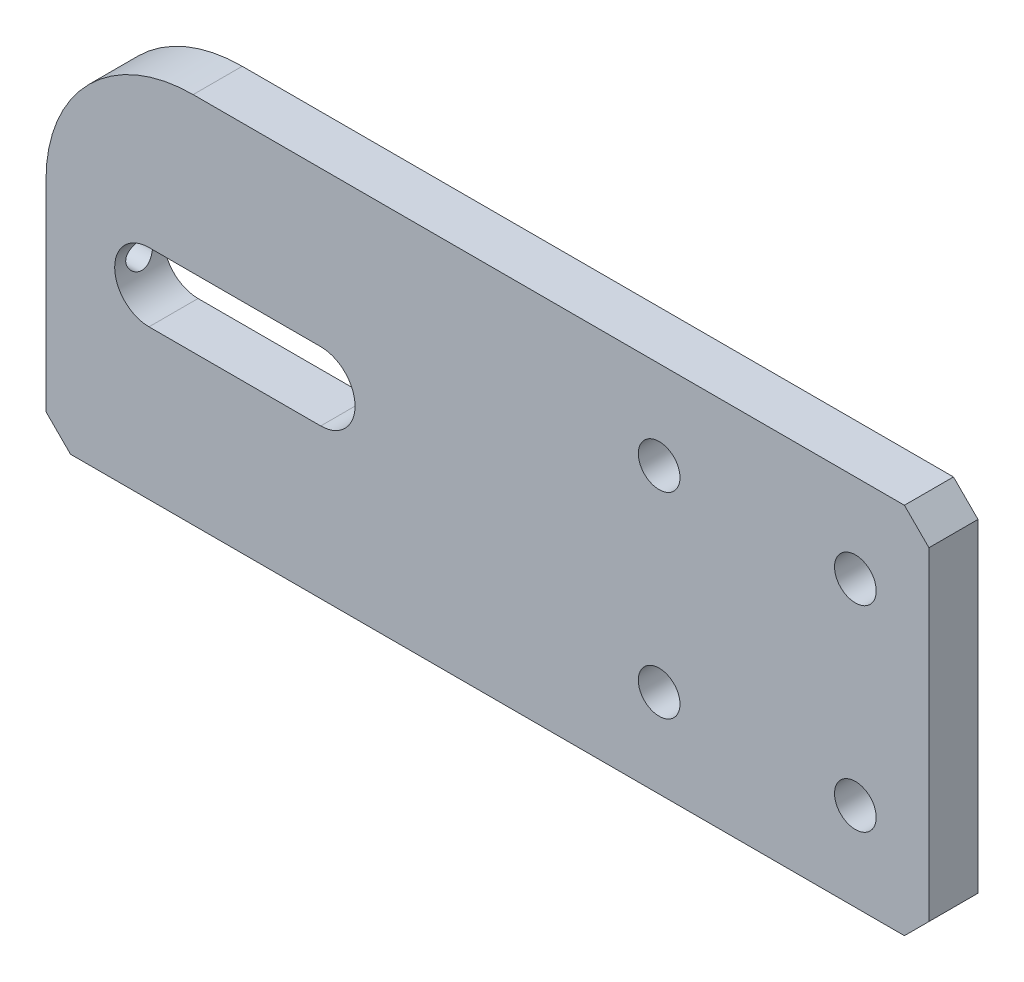
SolidWorks part; units mm, degrees
ref_plane "前视基准面" through (0, 0, 0) normal (0, 0, 1) x (1, 0, 0)
ref_plane "上视基准面" through (0, 0, 0) normal (0, 1, 0) x (1, 0, 0)
ref_plane "右视基准面" through (0, 0, 0) normal (1, 0, 0) x (0, 0, -1)
sketch "草图2" plane through (0, 0, 0) normal (0, 0, 1) x (1, 0, 0)
  line L1 (-60, 38) -> (90, 38)
  line L2 (-90, 8) -> (-90, -38)
  line L3 (-90, -38) -> (90, -38)
  line L4 (90, 38) -> (90, -38)
  line L5 (-90, 38) -> (90, -38) construction
  line L6 (-90, -38) -> (90, 38) construction
  arc A0 (-90, 8) -> (-60, 38) centre (-60, 8) cw
  point P0 (0, 0)
  dimension "D3" = 30
  dimension "D1" = 180
  dimension "D2" = 76
extrude "凸台-拉伸1" add sketch "草图2" along normal mid plane 10
hole_wizard "Ø8.5 (8.5) 直径孔1" positions "草图4" profile "草图3" hole size "Ø8.5" standard "GB" end condition through all
sketch "草图4" plane through (0, 0, 5) normal (0, 0, 1) x (1, 0, 0)
  line L0 (90, -38) -> (90, 38) construction
  point P0 (75, 20)
  dimension "D1" = 20
  dimension "D2" = 15
sketch "草图3" plane through (75, 20, 5) normal (1, 0, 0) x (0, -1, 0)
  line L0 (0, 0) -> (0, 10)
  line L1 (0, 10) -> (4.25, 10)
  line L2 (4.25, 10) -> (4.25, 0)
  line L5 (4.25, 0) -> (0, 0)
  line L11 (0, -6.35) -> (0, 107.95) construction
  dimension "通孔孔直径" = 8.5
  dimension "通孔孔深度" = 10
pattern_linear "阵列(线性)1" count 2 spacing 40 along (-1, 0, 0) of "Ø8.5 (8.5) 直径孔1"
mirror "镜向1" about plane through (0, 0, 0) normal (0, 1, 0) of "阵列(线性)1", "Ø8.5 (8.5) 直径孔1"
sketch "草图5" plane through (0, 0, 5) normal (0, 0, 1) x (1, 0, 0)
  line L0 (-69, -0.5) -> (-34, -0.5) construction
  line L1 (-69, 6.5) -> (-34, 6.5)
  line L2 (-69, -7.5) -> (-34, -7.5)
  line L3 (-90, -38) -> (90, -38) construction
  line L4 (-90, 8) -> (-90, -38) construction
  arc A0 (-69, 6.5) -> (-69, -7.5) centre (-69, -0.5) ccw
  arc A1 (-34, -7.5) -> (-34, 6.5) centre (-34, -0.5) ccw
  point P2 (-51.5, -0.5)
  dimension "D4" = 21
  dimension "D1" = 14
  dimension "D2" = 35
  dimension "D3" = 37.5
extrude "切除-拉伸1" cut sketch "草图5" against normal blind 10
hole_wizard "Ø5.5 (5.5) 直径孔1" positions "草图7" profile "草图6" hole size "Ø5.5" standard "GB"
sketch "草图7" plane through (-90, 0, 0) normal (-1, 0, 0) x (0, 0, 1)
  line L0 (5, -38) -> (-5, -38) construction
  point P0 (0, -0.5)
  dimension "D1" = 37.5
sketch "草图6" plane through (-90, -0.5, 0) normal (0, 1, 0) x (0, 0, 1)
  line L0 (0, 0) -> (0, 14)
  line L1 (0, 14) -> (2.75, 14)
  line L2 (2.75, 14) -> (2.75, 0)
  line L5 (2.75, 0) -> (0, 0)
  line L11 (0, -6.35) -> (0, 107.95) construction
  dimension "通孔孔直径" = 5.5
  dimension "通孔孔深度" = 14
chamfer "倒角1" distance 5 angle 45 3 edges at (90, 38, 0) (90, -38, 0) (-90, -38, 0)
